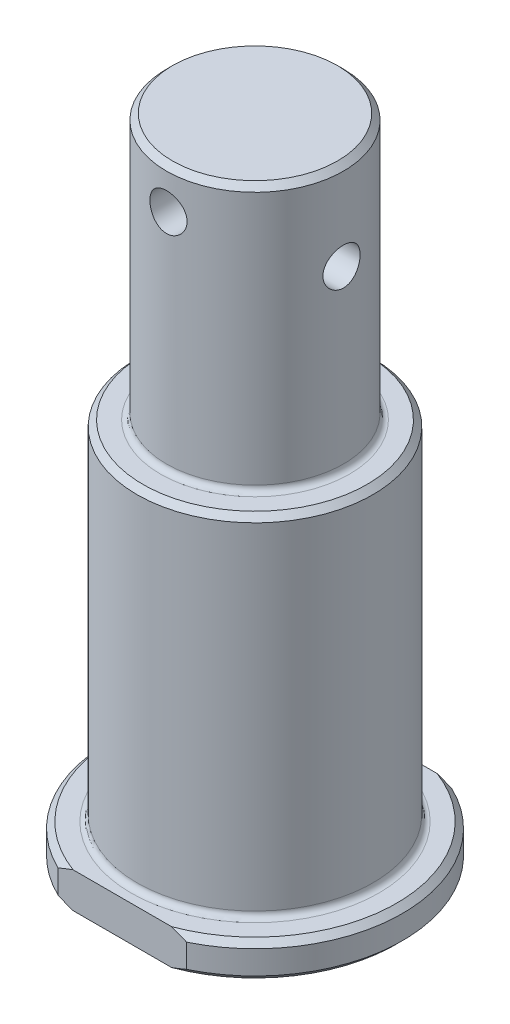
SolidWorks part; units mm, degrees
material "45#"
ref_plane "Front Plane" through (0, 0, 0) normal (0, 0, 1) x (1, 0, 0)
ref_plane "Top Plane" through (0, 0, 0) normal (0, 1, 0) x (1, 0, 0)
ref_plane "Right Plane" through (0, 0, 0) normal (1, 0, 0) x (0, 0, -1)
sketch "Sketch1" plane through (0, 0, 0) normal (0, 0, 1) x (1, 0, 0)
  line L0 (0, 0) -> (25, 0)
  line L1 (25, 0) -> (25, 6)
  line L2 (25, 6) -> (20, 6)
  line L3 (20, 6) -> (20, 65)
  line L4 (20, 65) -> (15, 65)
  line L5 (15, 65) -> (15, 110)
  line L6 (15, 110) -> (0, 110)
  line L7 (0, 110) -> (0, 0)
  line L8 (0, 0) -> (0, -9.4882) construction
  dimension "D1" = 50
  dimension "D2" = 40
  dimension "D3" = 30
  dimension "D4" = 110
  dimension "D5" = 45
  dimension "D6" = 59
revolve "Revolve1" add sketch "Sketch1" angle 360 about L8
cosmetic thread "Cosmetic Thread1" parameters "D1"=44, "D2"=26.211
chamfer "Chamfer1" distance 1 angle 45 4 edges at (0, 0, 25) (0, 6, 25) (0, 110, 15) (0, 65, 20)
fillet "Fillet1" radius 1 2 edges at (0, 65, 15) (0, 6, 20)
sketch "Sketch2" plane through (0, 0, 0) normal (0, 1, 0) x (1, 0, 0)
  line L1 (40, -22.5) -> (-40, -22.5)
  line L2 (40, -22.5) -> (40, 22.5)
  line L3 (40, 22.5) -> (-40, 22.5)
  line L4 (-40, -22.5) -> (-40, 22.5)
  line L5 (40, -22.5) -> (-40, 22.5) construction
  line L6 (40, 22.5) -> (-40, -22.5) construction
  point P0 (0, 0)
  dimension "D1" = 45
  dimension "D2" = 80
extrude "Cut-Extrude1" cut sketch "Sketch2" along normal up to surface (6 mm away) flip side to cut up to face at (0, 6, -21)
sketch "Sketch3" plane through (0, 0, 0) normal (0, 0, 1) x (1, 0, 0)
  line L0 (0, 110) -> (0, 103) construction
  line L1 (14, 110) -> (-14, 110) construction
  circle A0 centre (0, 103) radius 3.15
  dimension "D2" = 6.3
  dimension "D1" = 7
extrude "Cut-Extrude2" cut sketch "Sketch3" against normal through all both and the other way through all
sketch "Sketch4" plane through (0, 0, 0) normal (1, 0, 0) x (0, 0, -1)
  line L0 (0, 110) -> (0, 95) construction
  line L1 (14, 110) -> (-14, 110) construction
  circle A0 centre (0, 95) radius 3.15
  dimension "D2" = 6.3
  dimension "D1" = 15
extrude "Cut-Extrude3" cut sketch "Sketch4" against normal through all both and the other way through all
